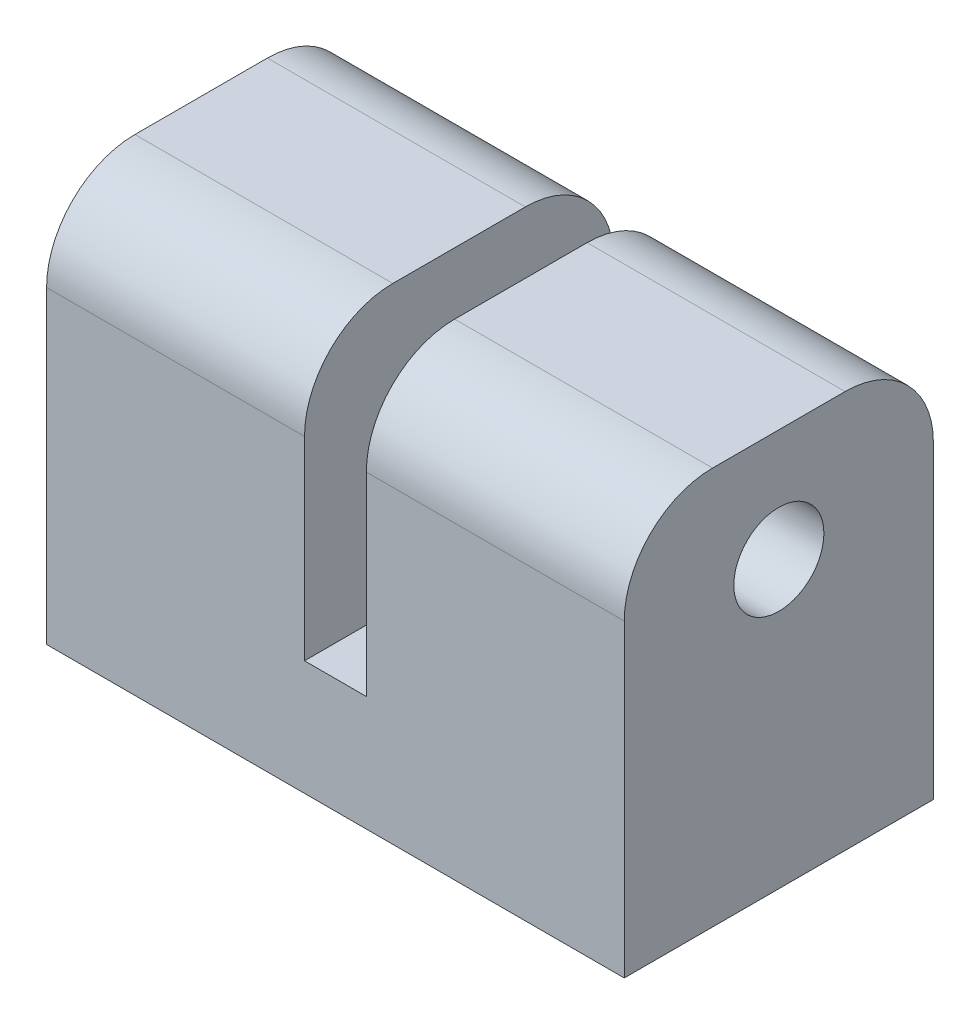
from build123d import *

# Parameters (mm, degrees)
SKETCH_1_W          = 65.4
SKETCH_1_H          = 45
EXTRUDE_1_DEPTH     = 35
FILLET_1_R          = 10
SKETCH_2_R          = 5.1
CUT_EXTRUDE_1_DEPTH = 84
SKETCH_3_W          = 7
SKETCH_3_H          = 50
CUT_EXTRUDE_2_DEPTH = 35


with BuildPart() as part:
    # 草图1 → 凸台-拉伸1 (new body)
    with BuildSketch(Plane.XY):
        Rectangle(SKETCH_1_W, SKETCH_1_H)
    extrude(amount=EXTRUDE_1_DEPTH)

    # 圆角1
    fillet_1_edges = [part.edges().sort_by_distance(p)[0] for p in [
        (0, 22.5, 35),
        (0, 22.5, 0),
    ]]
    fillet(fillet_1_edges, radius=FILLET_1_R)

    # 草图2 → 切除-拉伸1 (cut)
    with BuildSketch(Plane(origin=(32.7, 0, 0), x_dir=(0, 0, -1), z_dir=(1, 0, 0))):
        with Locations((-17.5, 9.8)):
            Circle(SKETCH_2_R)
    extrude(amount=-CUT_EXTRUDE_1_DEPTH, mode=Mode.SUBTRACT)

    # 草图3 → 切除-拉伸2 (cut)
    with BuildSketch(Plane.XY.offset(35)):
        with Locations((0, 15.5)):
            Rectangle(SKETCH_3_W, SKETCH_3_H)
    extrude(amount=-CUT_EXTRUDE_2_DEPTH, mode=Mode.SUBTRACT)


solid = part.part
